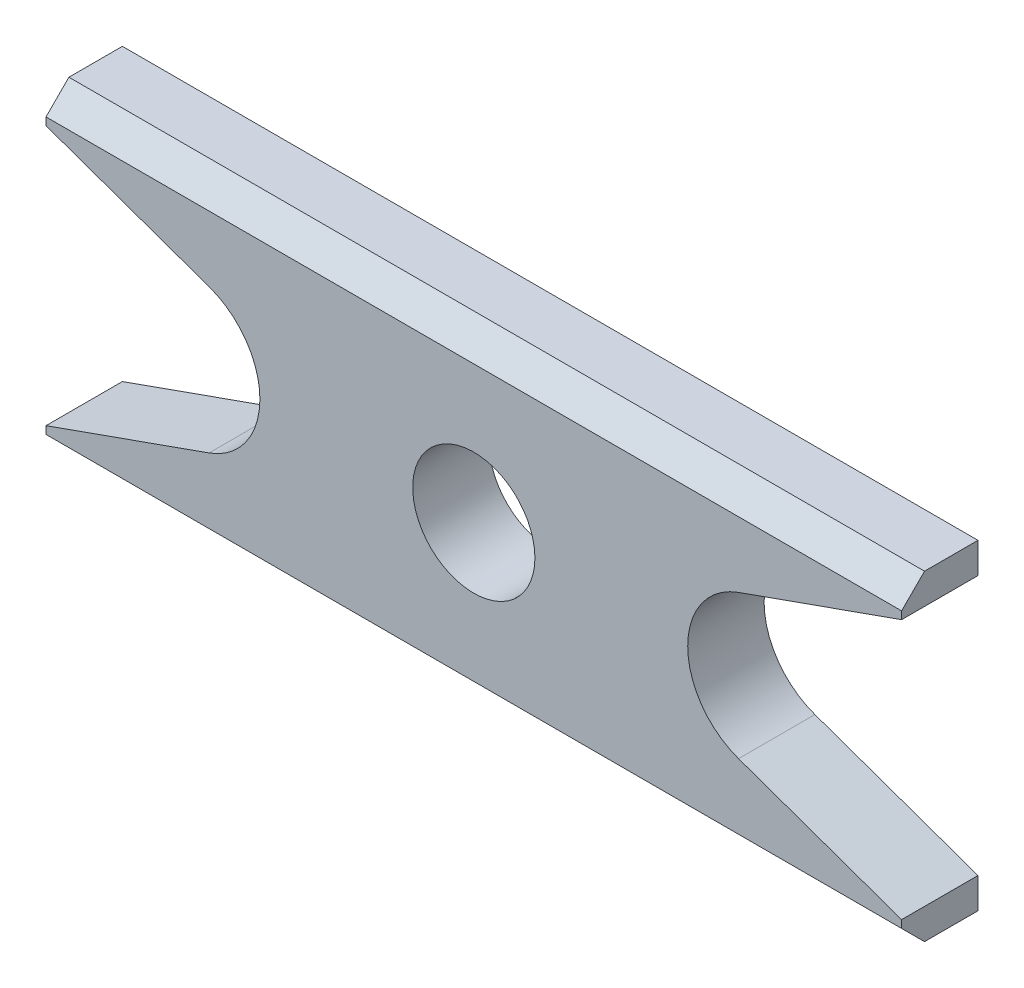
SolidWorks part; units mm, degrees
material "Q235-A"
ref_plane "Front Plane" through (0, 0, 0) normal (0, 0, 1) x (1, 0, 0)
ref_plane "Top Plane" through (0, 0, 0) normal (0, 1, 0) x (1, 0, 0)
ref_plane "Right Plane" through (0, 0, 0) normal (1, 0, 0) x (0, 0, -1)
sketch "Sketch1" plane through (0, 0, 0) normal (0, 0, 1) x (1, 0, 0)
  line L0 (0, -378.8368) -> (0, 378.8368) construction
  line L1 (190, 0) -> (-190, 0) construction
  line L2 (-280, 105) -> (280, 105)
  line L3 (280, 105) -> (280, 85)
  line L4 (280, 85) -> (173.2756, 47.12)
  line L5 (280, -85) -> (173.2756, -47.12)
  line L6 (280, -105) -> (280, -85)
  line L7 (-280, -105) -> (280, -105)
  line L8 (-280, -105) -> (-280, -85)
  line L9 (-280, -85) -> (-173.2756, -47.12)
  line L10 (-280, 85) -> (-173.2756, 47.12)
  line L11 (-280, 105) -> (-280, 85)
  circle A0 centre (0, 0) radius 40
  arc A1 (173.2756, 47.12) -> (173.2756, -47.12) centre (190, 0) ccw
  arc A2 (-173.2756, 47.12) -> (-173.2756, -47.12) centre (-190, 0) cw
  point P4 (0, 0)
  point P8 (0, 0)
  point P21 (0, -105)
  point P22 (0, 0)
  point P25 (0, 105)
  dimension "D1" = 80
  dimension "D2" = 100
  dimension "D3" = 280
  dimension "D4" = 210
  dimension "D5" = 20
  dimension "D6" = 90
extrude "Boss-Extrude1" add sketch "Sketch1" along normal mid plane 50
chamfer "Chamfer1" distance 15 angle 45 2 edges at (0, -105, 25) (0, 105, 25)
